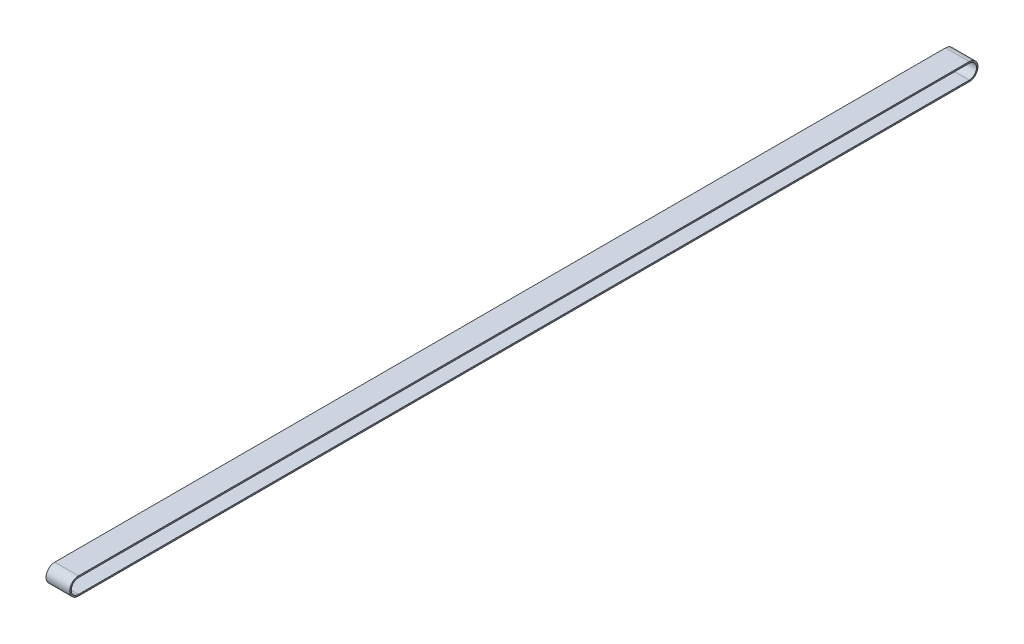
SolidWorks part; units mm, degrees
ref_plane "前基準面" through (0, 0, 0) normal (0, 0, 1) x (1, 0, 0)
ref_plane "上基準面" through (0, 0, 0) normal (0, 1, 0) x (1, 0, 0)
ref_plane "右基準面" through (0, 0, 0) normal (1, 0, 0) x (0, 0, -1)
sketch "草图1" plane through (0, 0, 0) normal (1, 0, 0) x (0, 0, -1)
  line L0 (0, 0) -> (3002.5, 0) construction
  line L1 (0, 27.325) -> (3002.5, 27.325)
  line L2 (0, -27.325) -> (3002.5, -27.325)
  arc A1 (0, 27.325) -> (0, -27.325) centre (0, 0) ccw
  arc A2 (3002.5, -27.325) -> (3002.5, 27.325) centre (3002.5, 0) ccw
  point P3 (1501.25, 0)
  dimension "D1" = 54.65
  dimension "D2" = 3002.5
extrude "拉伸-薄壁1" add sketch "草图1" along normal mid plane 80 thin thin type one direction wall 2.25
sketch "草图2" plane through (0, 0, 0) normal (1, 0, 0) x (0, 0, -1)
  line L2 (3002.5, 27.325) -> (0, 27.325)
  line L3 (0, -27.325) -> (3002.5, -27.325)
  line L4 (3002.5, 27.325) -> (0, 27.325)
  line L5 (0, -27.325) -> (3002.5, -27.325)
  arc A2 (3002.5, -27.325) -> (3002.5, 27.325) centre (3002.5, 0) ccw
  arc A3 (0, 27.325) -> (0, -27.325) centre (0, 0) ccw
  arc A4 (3002.5, -27.325) -> (3002.5, 27.325) centre (3002.5, 0) ccw
  arc A5 (0, 27.325) -> (0, -27.325) centre (0, 0) ccw
  dimension "D1" = 0
extrude "拉伸-薄壁2" add sketch "草图2" along normal mid plane 80 separate body thin thin type one direction reverse wall 2.83
